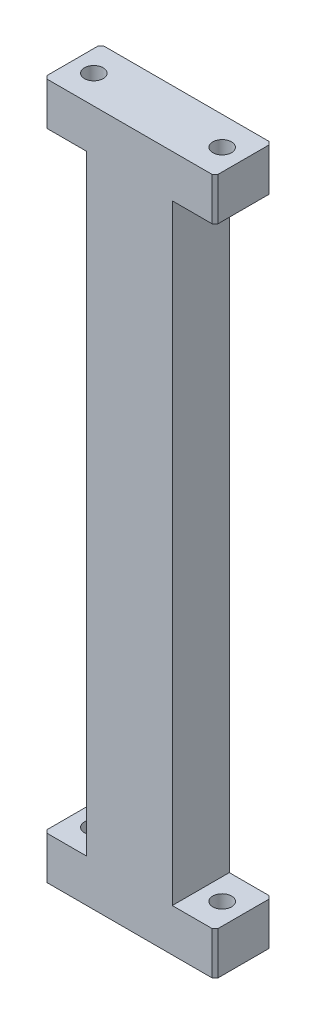
SolidWorks part; units mm, degrees
material "6061 合金"
ref_plane "Front Plane" through (0, 0, 0) normal (0, 0, 1) x (1, 0, 0)
ref_plane "Top Plane" through (0, 0, 0) normal (0, 1, 0) x (1, 0, 0)
ref_plane "Right Plane" through (0, 0, 0) normal (1, 0, 0) x (0, 0, -1)
sketch "Sketch1" plane through (0, 0, 0) normal (0, 0, 1) x (1, 0, 0)
  line L1 (-30, 122) -> (30, 122)
  line L2 (-30, 122) -> (-30, -122)
  line L3 (-30, -122) -> (30, -122)
  line L4 (30, 122) -> (30, -122)
  line L5 (-30, 122) -> (30, -122) construction
  line L6 (-30, -122) -> (30, 122) construction
  point P0 (0, 0)
  dimension "D1" = 60
  dimension "D2" = 244
extrude "Boss-Extrude1" add sketch "Sketch1" along normal blind 20
sketch "Sketch2" plane through (0, 0, 20) normal (0, 0, 1) x (1, 0, 0)
  line L0 (-30, 122) -> (-30, -122) construction
  line L1 (-30, 107) -> (-15, 107)
  line L2 (-30, 107) -> (-30, -107)
  line L3 (-30, -107) -> (-15, -107)
  line L4 (-15, 107) -> (-15, -107)
  line L5 (30, -122) -> (30, 122) construction
  line L6 (30, 107) -> (15, 107)
  line L7 (30, 107) -> (30, -107)
  line L8 (30, -107) -> (15, -107)
  line L9 (15, 107) -> (15, -107)
  line L10 (0, 0) -> (15, 0) construction
  line L11 (30, 122) -> (-30, 122) construction
  dimension "D1" = 15
  dimension "D2" = 15
extrude "Cut-Extrude1" cut sketch "Sketch2" against normal through all
hole_wizard "M6 Clearance Hole1" positions "Sketch3" profile "Sketch4" hole size "M6" standard "ISO" end condition through all
sketch "Sketch3" plane through (0, 122, 0) normal (0, 1, 0) x (1, 0, 0)
  line L0 (-30, -10) -> (-22.5, -10) construction
  line L1 (-30, -20) -> (-30, 0) construction
  line L3 (30, -20) -> (30, 0) construction
  point P0 (-22.5, -10)
  point P2 (22.5, -10)
  dimension "D1" = 7.5
  dimension "D2" = 7.5
sketch "Sketch4" plane through (-22.5, 122, 10) normal (1, 0, 0) x (0, 0, 1)
  line L0 (0, 0) -> (0, 244)
  line L1 (0, 244) -> (3.3, 244)
  line L2 (3.3, 244) -> (3.3, 0)
  line L5 (3.3, 0) -> (0, 0)
  line L11 (0, -6.35) -> (0, 107.95) construction
  dimension "通孔孔直径" = 6.6
  dimension "通孔孔深度" = 244
chamfer "Chamfer1" distance 1 angle 45 8 edges at (-30, -114.5, 20) (-30, -114.5, 0) (30, -114.5, 0) (30, -114.5, 20) (30, 114.5, 20) (30, 114.5, 0) (-30, 114.5, 0) (-30, 114.5, 20)
